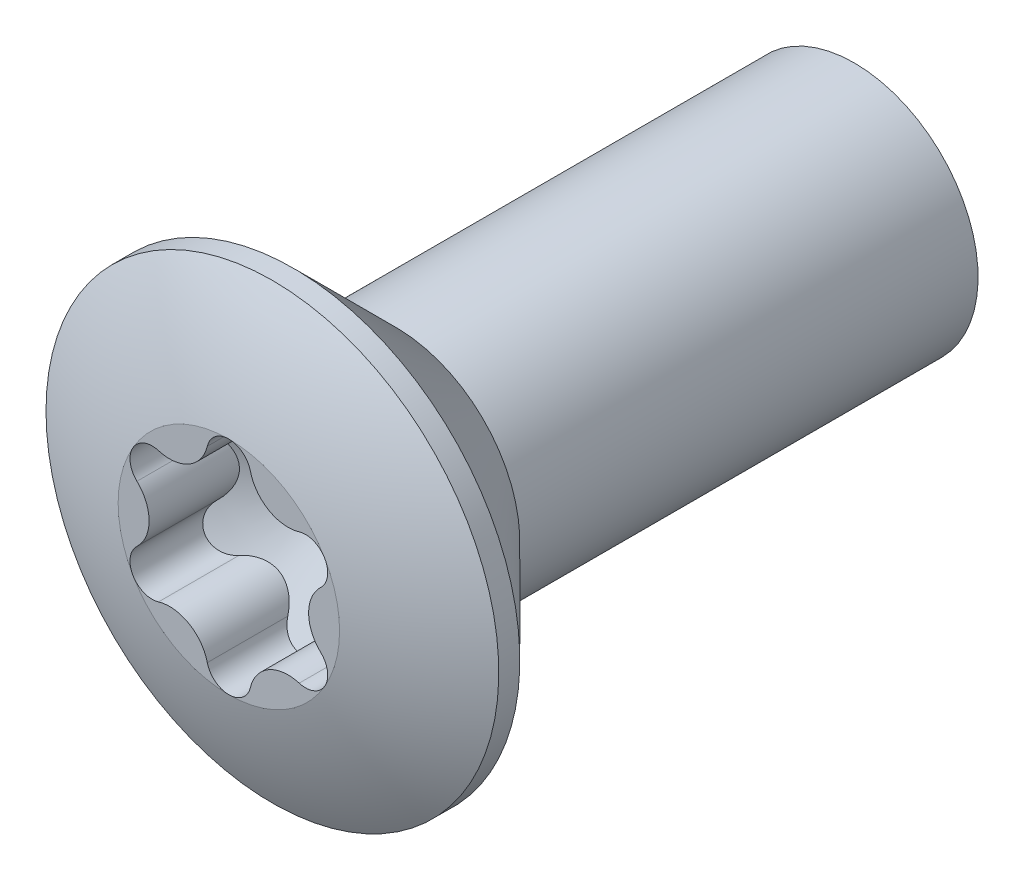
SolidWorks part; units mm, degrees
ref_plane "Front Plane" through (0, 0, 0) normal (0, 0, 1) x (1, 0, 0)
ref_plane "Top Plane" through (0, 0, 0) normal (0, 1, 0) x (1, 0, 0)
ref_plane "Right Plane" through (0, 0, 0) normal (1, 0, 0) x (0, 0, -1)
other "Configuration Table"
sketch "BodySke" plane through (0, 0, 0) normal (1, 0, 0) x (0, 0, -1)
  line L0 (0, 0) -> (-1787.2758, 0) construction
  line L2 (3.13, 9.15) -> (7.28, 5)
  line L4 (7.28, 5) -> (26.28, 5)
  line L5 (26.28, 5) -> (26.28, 0)
  line L6 (26.28, 0) -> (0, 0)
  line L7 (-3.72, 7.25) -> (-3.72, 50007.25) construction
  line L8 (3.13, 9.15) -> (2.28, 9.15)
  arc A0 (0, 0) -> (2.28, 9.15) centre (19.5, 0) cw
  point P18 (2.705, 9.15)
revolve "Base-Revolve" add sketch "BodySke" angle 360 about L0
cosmetic thread "ThreadCosmetic" [suppressed] parameters "ThdLen"=30, "MinorDia"=8.344
sketch "PreBSke" plane through (0, 0, 0) normal (1, 0, 0) x (0, 0, -1)
  line L0 (0, 0) -> (-50000, 0) construction
  line L1 (0, 0) -> (0, 4.475)
  line L3 (0, 4.475) -> (3.42, 4.475)
  line L4 (3.42, 4.475) -> (6.1089, 0)
  line L5 (6.1089, 0) -> (0, 0)
  line L6 (3.42, -4.475) -> (6.1089, 0) construction
revolve "PreBroach" cut sketch "PreBSke" angle 360 about L0
ref_plane "Plane1" through (0, 0, -0.5204) normal (0, 0, 1) x (1, 0, 0)
sketch "HexSke" plane through (0, 0, -0.5204) normal (0, 0, 1) x (1, 0, 0)
  line L0 (0, 0) -> (-42905.1683, 24771.3105) construction
  line L1 (0, 0) -> (-42905.1683, -24771.3105) construction
  line L2 (0, 0) -> (50000, 0) construction
  arc A0 (-3.7147, -1.1391) -> (-3.7147, 1.1391) centre (-4.7896, 0) ccw
  arc A1 (-3.8755, 2.2375) -> (-3.7147, 1.1391) centre (-3.1004, 1.79) ccw
  arc A2 (-3.7147, -1.1391) -> (-3.8755, -2.2375) centre (-3.1004, -1.79) ccw
  arc A3 (-2.8438, 2.6474) -> (-3.8755, 2.2375) centre (-3.1004, 1.79) ccw
  circle A4 centre (0, 0) radius 3.2234 construction
  circle A5 centre (0, 0) radius 4.475 construction
  arc A6 (-2.8438, 2.6474) -> (-0.8708, 3.7865) centre (-2.3948, 4.148) ccw
  arc A7 (0, 4.475) -> (-0.8708, 3.7865) centre (0, 3.58) ccw
  arc A8 (0.8708, 3.7865) -> (0, 4.475) centre (0, 3.58) ccw
  arc A9 (0.8708, 3.7865) -> (2.8438, 2.6474) centre (2.3948, 4.148) ccw
  arc A10 (3.8755, 2.2375) -> (2.8438, 2.6474) centre (3.1004, 1.79) ccw
  arc A11 (3.7147, 1.1391) -> (3.8755, 2.2375) centre (3.1004, 1.79) ccw
  arc A12 (3.7147, 1.1391) -> (3.7147, -1.1391) centre (4.7896, 0) ccw
  arc A13 (3.8755, -2.2375) -> (3.7147, -1.1391) centre (3.1004, -1.79) ccw
  arc A14 (2.8438, -2.6474) -> (3.8755, -2.2375) centre (3.1004, -1.79) ccw
  arc A15 (2.8438, -2.6474) -> (0.8708, -3.7865) centre (2.3948, -4.148) ccw
  arc A16 (0, -4.475) -> (0.8708, -3.7865) centre (0, -3.58) ccw
  arc A17 (-0.8708, -3.7865) -> (0, -4.475) centre (0, -3.58) ccw
  arc A18 (-0.8708, -3.7865) -> (-2.8438, -2.6474) centre (-2.3948, -4.148) ccw
  arc A19 (-3.8755, -2.2375) -> (-2.8438, -2.6474) centre (-3.1004, -1.79) ccw
  circle A21 centre (0, 0) radius 4.475
  point P56 (0, 0)
extrude "Hexalobular" add sketch "HexSke" against normal up to next
sketch "ThdSchSke" plane through (0, 0, 0) normal (1, 0, 0) x (0, 0, -1)
  line L0 (26.7581, 5) -> (26.28, 4.172)
  line L1 (26.28, 4.172) -> (25.802, 5)
  line L2 (25.802, 5) -> (26.7581, 5)
  line L3 (26.28, 4.172) -> (26.28, 5) construction
  line L4 (26.28, -5) -> (26.28, 5) construction
  line L5 (26.28, 5) -> (7.28, 5) construction
  line L6 (0, 0) -> (-50000, 0) construction
revolve "ThreadSchematic" cut sketch "ThdSchSke" angle 360 about L6
ref_plane "ThreadPlane" through (0, 0, 3.72) normal (0, 0, -1) x (-1, 0, 0)
pattern_linear "ThdSchPat" [suppressed] count 12
equation "\"Ri@HexSke\"= .1 * \"A@PreBSke\""
equation "\"Re@HexSke\"= .175 * \"A@PreBSke\""
equation "\"MinorDia@ThreadCosmetic\"= \"MinorDia@ThdSchSke\""
equation "\"ThreadLength\"= IIF ( \"B@BodySke\" = \"L@BodySke\" , \"L@BodySke\" - \"K@BodySke\" , \"B@BodySke\" )"
equation "\"ThdLen@ThreadPlane\"=\"ThreadLength\""
equation "\"ThdLen@ThreadCosmetic\"=\"ThreadLength\""
